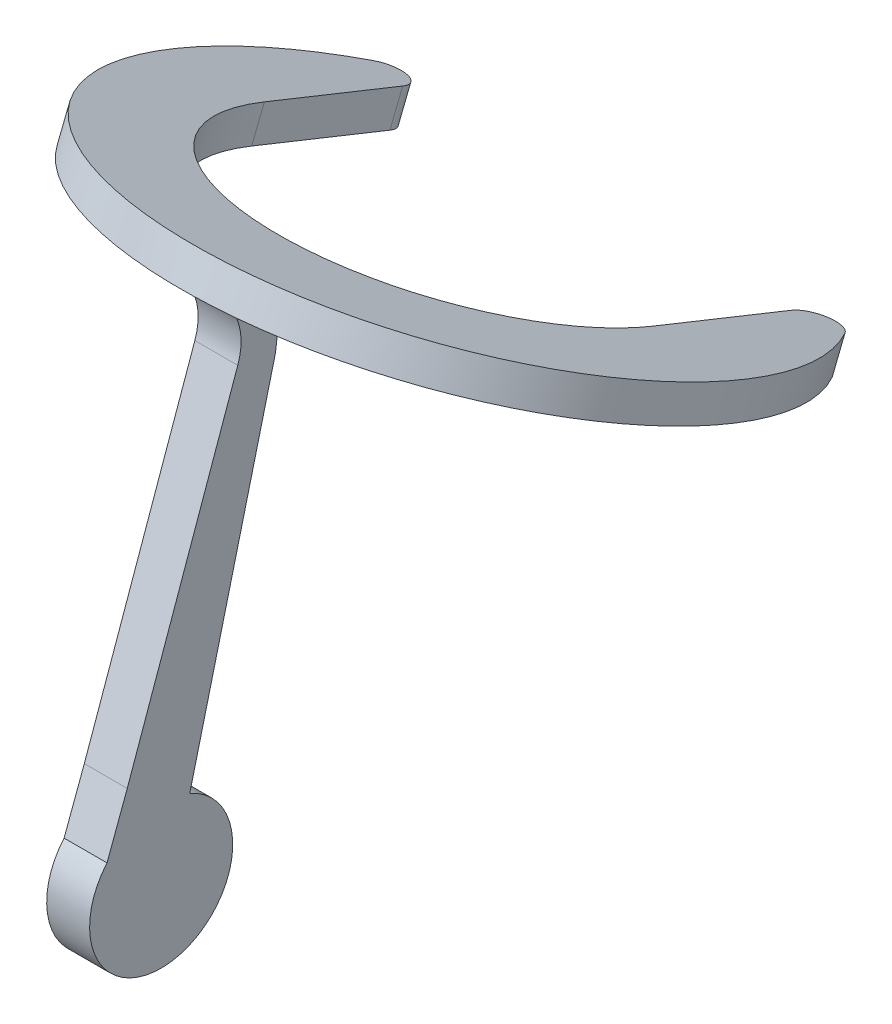
SolidWorks part; units mm, degrees
ref_plane "Front Plane" through (0, 0, 0) normal (0, 0, 1) x (1, 0, 0)
ref_plane "Top Plane" through (0, 0, 0) normal (0, 1, 0) x (1, 0, 0)
ref_plane "Right Plane" through (0, 0, 0) normal (1, 0, 0) x (0, 0, -1)
sketch "Sketch1" plane through (0, 0, 0) normal (1, 0, 0) x (0, 0, -1)
  circle A0 centre (0, 0) radius 25
  dimension "D1" = 50
extrude "Boss-Extrude1" add sketch "Sketch1" along normal mid plane 15
sketch "Sketch2" plane through (0, 0, 0) normal (1, 0, 0) x (0, 0, -1)
  line L0 (-25, 0) -> (-11.8529, 35.3339)
  line L1 (-11.8529, 35.3339) -> (33.1975, 162.1534)
  line L2 (-25, 0) -> (3.6658, -1.9997)
  line L3 (3.6658, -1.9997) -> (39.9174, 141.1253)
  line L4 (39.9174, 141.1253) -> (42.1154, 158.5807)
  line L5 (42.1154, 158.5807) -> (33.1975, 162.1534)
  circle A0 centre (0, 0) radius 25 construction
extrude "Boss-Extrude2" add sketch "Sketch2" along normal mid plane 15
sketch "Sketch4" plane through (0, 151.1876, -60.5693) normal (0, 0.9283, -0.3719) x (1, 0, 0)
  line L0 (67.8521, 102.0293) -> (67.8521, 49.9672)
  line L1 (0, -57.7577) -> (0, 91.8025) construction
  line L2 (-67.8521, 102.0293) -> (-67.8521, 49.9672)
  arc A0 (-82.4479, 106.5565) -> (82.4479, 106.5565) centre (0, 49.9672) ccw
  arc A1 (-67.8521, 49.9672) -> (67.8521, 49.9672) centre (0, 49.9672) ccw
  circle A2 centre (0, 49.9672) radius 67.8521 construction
  circle A3 centre (0, 49.9672) radius 100 construction
  arc A4 (-67.8521, 102.0293) -> (-82.4479, 106.5565) centre (-75.8521, 102.0293) ccw
  arc A5 (67.8521, 102.0293) -> (82.4479, 106.5565) centre (75.8521, 102.0293) cw
  point P13 (-67.8521, 123.4253)
  point P16 (67.8521, 123.4253)
  dimension "D1" = 200
  dimension "D2" = 8
extrude "Boss-Extrude4" add sketch "Sketch4" along normal blind 12
fillet "Fillet1" radius 20 1 edges at (0, 162.1534, -33.1975)
